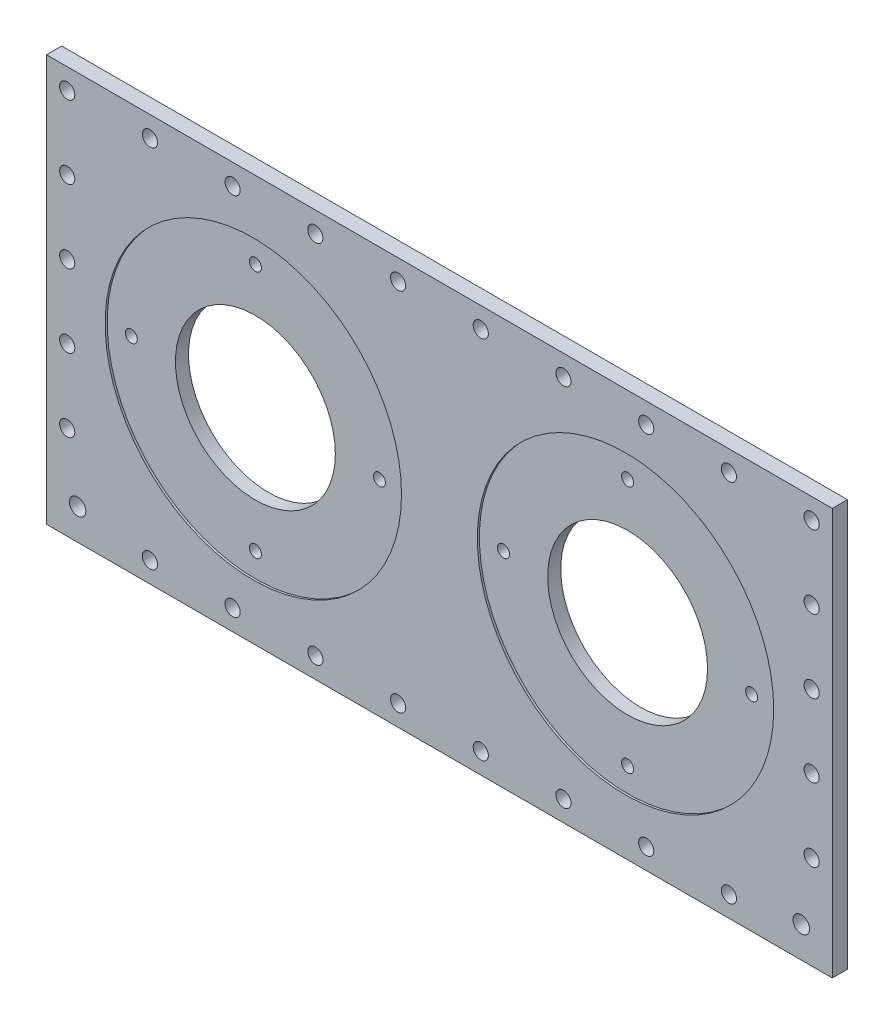
from build123d import *

# Parameters (mm, degrees)
SKETCH1_W           = 1140
SKETCH1_H           = 590
BOSS_EXTRUDE1_DEPTH = 22
SKETCH2_R           = 11
SKETCH2_R_2         = 12
CUT_EXTRUDE1_DEPTH  = 32
SKETCH3_R           = 116
CUT_EXTRUDE2_DEPTH  = 32
SKETCH4_R           = 215
CUT_EXTRUDE3_DEPTH  = 3
CIRPATTERN1_COUNT   = 4
CIRCPATTERN2_COUNT  = 4


with BuildPart() as part:
    # Sketch1 → Boss-Extrude1 (new body)
    with BuildSketch(Plane.XY):
        with Locations((138.473053892, -23.233532934)):
            Rectangle(SKETCH1_W, SKETCH1_H)
    extrude(amount=BOSS_EXTRUDE1_DEPTH)

    # Sketch2 → Cut-Extrude1 (cut)
    with BuildSketch(Plane.XY.offset(22)):
        with Locations((-401.526946108, 241.766467066)):
            Circle(SKETCH2_R)
        with Locations((-281.526946108, 241.766467066)):
            Circle(SKETCH2_R)
        with Locations((-161.526946108, 241.766467066)):
            Circle(SKETCH2_R)
        with Locations((-41.526946108, 241.766467066)):
            Circle(SKETCH2_R)
        with Locations((78.473053892, 241.766467066)):
            Circle(SKETCH2_R)
        with Locations((198.473053892, 241.766467066)):
            Circle(SKETCH2_R)
        with Locations((318.473053892, 241.766467066)):
            Circle(SKETCH2_R)
        with Locations((438.473053892, 241.766467066)):
            Circle(SKETCH2_R)
        with Locations((558.473053892, 241.766467066)):
            Circle(SKETCH2_R)
        with Locations((678.473053892, 241.766467066)):
            Circle(SKETCH2_R)
        with Locations((-386.526946108, -273.233532934)):
            Circle(SKETCH2_R_2)
        with Locations((558.473053892, -288.233532934)):
            Circle(SKETCH2_R)
        with Locations((438.473053892, -288.233532934)):
            Circle(SKETCH2_R)
        with Locations((318.473053892, -288.233532934)):
            Circle(SKETCH2_R)
        with Locations((198.473053892, -288.233532934)):
            Circle(SKETCH2_R)
        with Locations((78.473053892, -288.233532934)):
            Circle(SKETCH2_R)
        with Locations((-41.526946108, -288.233532934)):
            Circle(SKETCH2_R)
        with Locations((-161.526946108, -288.233532934)):
            Circle(SKETCH2_R)
        with Locations((-281.526946108, -288.233532934)):
            Circle(SKETCH2_R)
        with Locations((663.473053892, -273.233532934)):
            Circle(SKETCH2_R_2)
        with Locations((-401.526946108, 135.766467066)):
            Circle(SKETCH2_R)
        with Locations((-401.526946108, 29.766467066)):
            Circle(SKETCH2_R)
        with Locations((-401.526946108, -76.233532934)):
            Circle(SKETCH2_R)
        with Locations((-401.526946108, -182.233532934)):
            Circle(SKETCH2_R)
        with Locations((678.473053892, -182.233532934)):
            Circle(SKETCH2_R)
        with Locations((678.473053892, -76.233532934)):
            Circle(SKETCH2_R)
        with Locations((678.473053892, 29.766467066)):
            Circle(SKETCH2_R)
        with Locations((678.473053892, 135.766467066)):
            Circle(SKETCH2_R)
    extrude(amount=-CUT_EXTRUDE1_DEPTH, mode=Mode.SUBTRACT)

    # Sketch3 → Cut-Extrude2 (cut)
    with BuildSketch(Plane.XY.offset(22)):
        with Locations((-131.526946108, -23.233532934)):
            Circle(SKETCH3_R)
        with Locations((408.473053892, -23.233532934)):
            Circle(SKETCH3_R)
    extrude(amount=-CUT_EXTRUDE2_DEPTH, mode=Mode.SUBTRACT)

    # Sketch4 → Cut-Extrude3 (cut)
    with BuildSketch(Plane.XY.offset(22)):
        with Locations((-131.526946108, -23.233532934)):
            Circle(SKETCH4_R)
        with Locations((408.473053892, -23.233532934)):
            Circle(SKETCH4_R)
    extrude(amount=-CUT_EXTRUDE3_DEPTH, mode=Mode.SUBTRACT)

    # Sketch6 → M20 Tapped Hole1 (revolve, cut)
    with BuildSketch(Plane(origin=(-131.526946108, 156.766467066, 19), x_dir=(0, -1, 0), z_dir=(1, 0, 0))):
        Polygon((0, 0), (0, 57.757530416), (8.75, 52.5), (8.75, 0), align=None)
    m20_tapped_hole1 = revolve(axis=Axis((-131.526946108, 156.766467066, 25.35), (0, 0, -1)), mode=Mode.SUBTRACT)

    # CirPattern1: M20 Tapped Hole1 ×4 about axis
    cirpattern1_axis = Axis((-131.526946108, -23.233532934, 0), (0, 0, 1))
    for i in range(1, CIRPATTERN1_COUNT):
        add(m20_tapped_hole1.rotate(cirpattern1_axis, i * 360 / CIRPATTERN1_COUNT), mode=Mode.SUBTRACT)

    # Sketch8 → M20 Tapped Hole2 (revolve, cut)
    with BuildSketch(Plane(origin=(408.473053892, 156.766467066, 19), x_dir=(0, -1, 0), z_dir=(1, 0, 0))):
        Polygon((0, 0), (0, 57.757530416), (8.75, 52.5), (8.75, 0), align=None)
    m20_tapped_hole2 = revolve(axis=Axis((408.473053892, 156.766467066, 25.35), (0, 0, -1)), mode=Mode.SUBTRACT)

    # CircPattern2: M20 Tapped Hole2 ×4 about axis
    circpattern2_axis = Axis((408.473053892, -23.233532934, 0), (0, 0, 1))
    for i in range(1, CIRCPATTERN2_COUNT):
        add(m20_tapped_hole2.rotate(circpattern2_axis, i * 360 / CIRCPATTERN2_COUNT), mode=Mode.SUBTRACT)


solid = part.part
